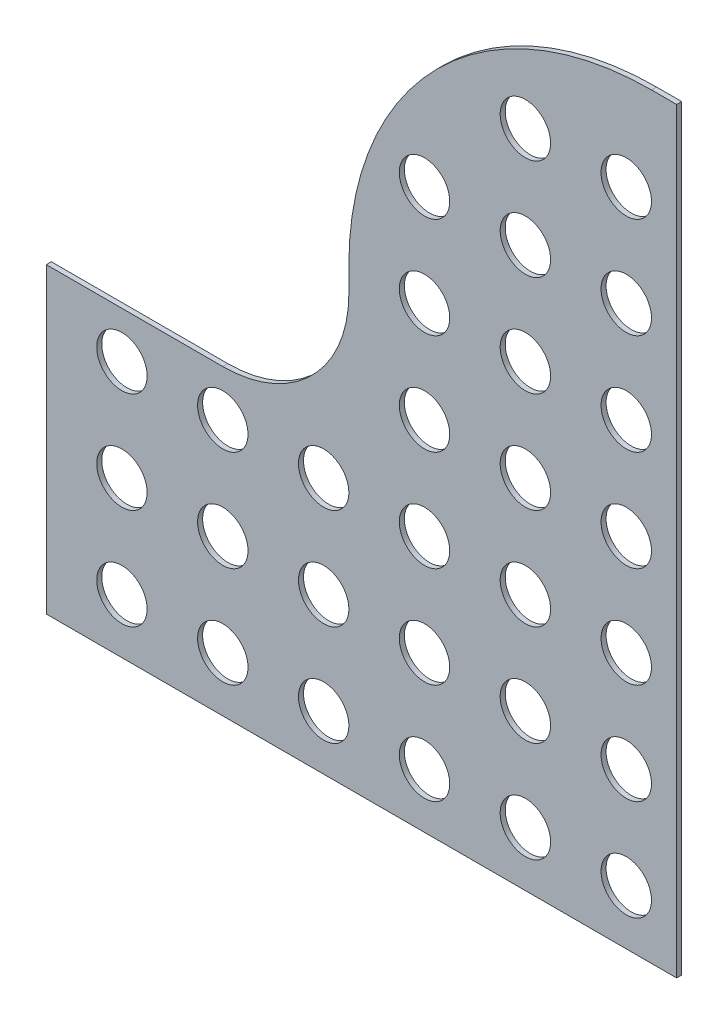
from build123d import *

# Parameters (mm, degrees)
BOSS_EXTRUDE1_DEPTH = 2
SKETCH2_R           = 10
CUT_EXTRUDE1_DEPTH  = 2


with BuildPart() as part:
    # Sketch1 → Boss-Extrude1 (new body)
    with BuildSketch(Plane.XY):
        with BuildLine():
            Line((0, 0), (250, 0))
            Line((250, 0), (250, 300))
            Line((250, 300), (240, 300))
            ThreePointArc((240, 300), (155.147186258, 264.852813742), (120, 180))
            Line((120, 180), (120, 170))
            ThreePointArc((120, 170), (105.355339059, 134.644660941), (70, 120))
            Line((70, 120), (0, 120))
            Line((0, 120), (0, 0))
        make_face()
    extrude(amount=BOSS_EXTRUDE1_DEPTH)

    # Sketch2 → Cut-Extrude1 (cut)
    with BuildSketch(Plane.XY.offset(2)):
        with Locations((230, 261.698838223)):
            Circle(SKETCH2_R)
        with Locations((190, 261.698838223)):
            Circle(SKETCH2_R)
        with Locations((230, 221.698838223)):
            Circle(SKETCH2_R)
        with Locations((190, 221.698838223)):
            Circle(SKETCH2_R)
        with Locations((230, 181.698838223)):
            Circle(SKETCH2_R)
        with Locations((190, 181.698838223)):
            Circle(SKETCH2_R)
        with Locations((230, 141.698838223)):
            Circle(SKETCH2_R)
        with Locations((190, 141.698838223)):
            Circle(SKETCH2_R)
        with Locations((230, 101.698838223)):
            Circle(SKETCH2_R)
        with Locations((190, 101.698838223)):
            Circle(SKETCH2_R)
        with Locations((230, 61.698838223)):
            Circle(SKETCH2_R)
        with Locations((190, 61.698838223)):
            Circle(SKETCH2_R)
        with Locations((230, 21.698838223)):
            Circle(SKETCH2_R)
        with Locations((190, 21.698838223)):
            Circle(SKETCH2_R)
        with Locations((150, 221.698838223)):
            Circle(SKETCH2_R)
        with Locations((150, 181.698838223)):
            Circle(SKETCH2_R)
        with Locations((150, 141.698838223)):
            Circle(SKETCH2_R)
        with Locations((150, 101.698838223)):
            Circle(SKETCH2_R)
        with Locations((150, 61.698838223)):
            Circle(SKETCH2_R)
        with Locations((150, 21.698838223)):
            Circle(SKETCH2_R)
        with Locations((110, 101.698838223)):
            Circle(SKETCH2_R)
        with Locations((70, 101.698838223)):
            Circle(SKETCH2_R)
        with Locations((30, 101.698838223)):
            Circle(SKETCH2_R)
        with Locations((110, 61.698838223)):
            Circle(SKETCH2_R)
        with Locations((70, 61.698838223)):
            Circle(SKETCH2_R)
        with Locations((30, 61.698838223)):
            Circle(SKETCH2_R)
        with Locations((110, 21.698838223)):
            Circle(SKETCH2_R)
        with Locations((70, 21.698838223)):
            Circle(SKETCH2_R)
        with Locations((30, 21.698838223)):
            Circle(SKETCH2_R)
    extrude(amount=-CUT_EXTRUDE1_DEPTH, mode=Mode.SUBTRACT)


solid = part.part
